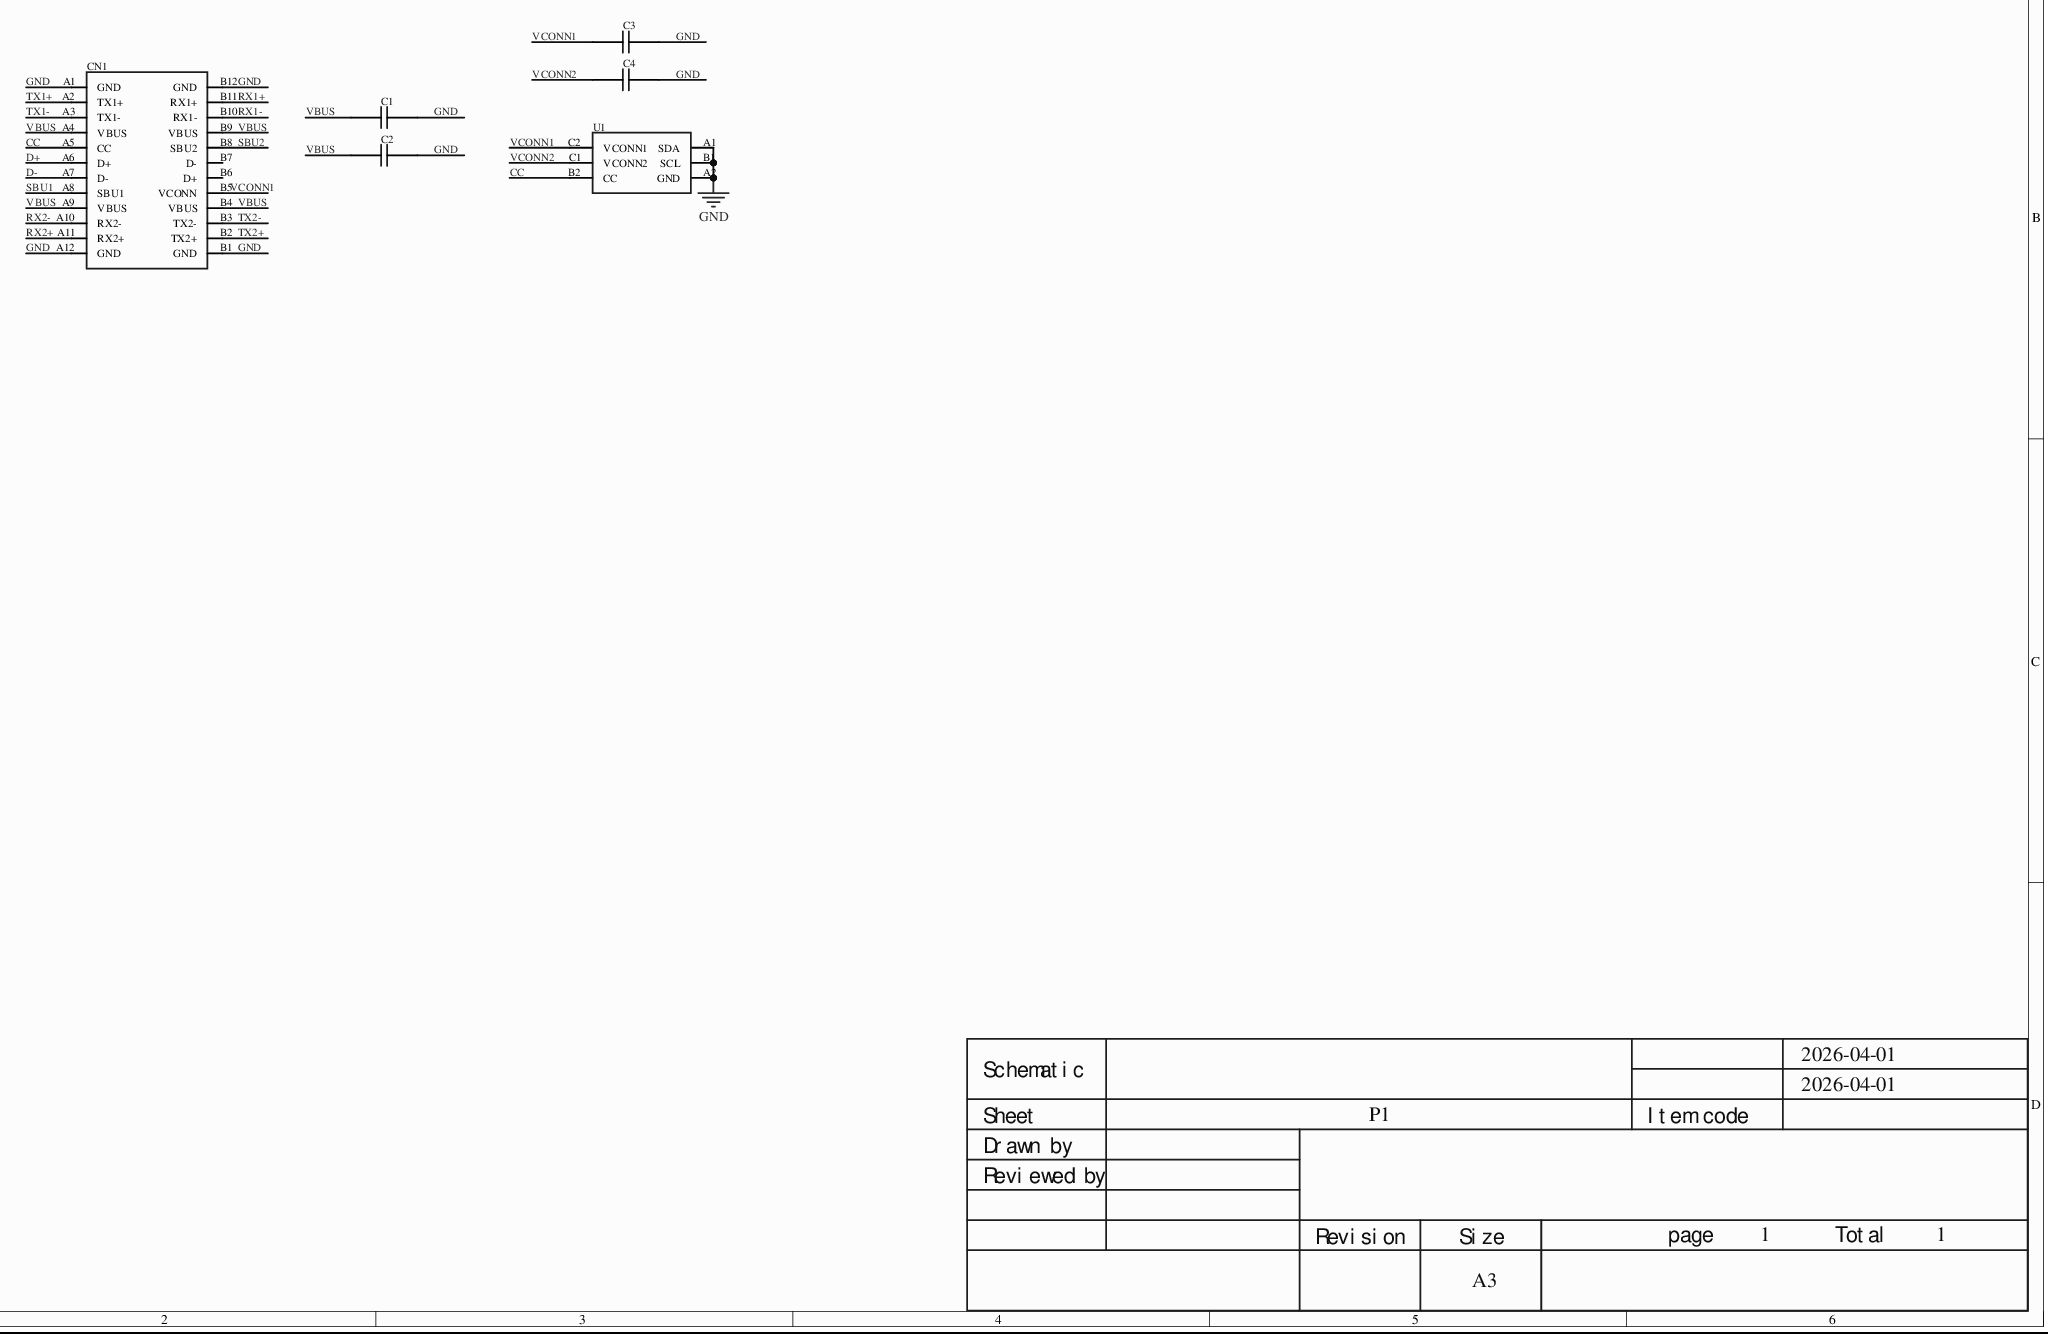
[diagram p0: MISC82881-3.schdoc]
# Altium project MISC82881-2.PrjPcb
1 sheet, 6 parts. Net scope: global (net labels, ports and power ports of the same name join across sheets).
Board file: MISC82881.pcbdoc

## Sheet MISC82881-3.schdoc
size 420 x 298 mm; Version: V1.0; @Project Name: MISC82881; @Page Count: 1; @Update Date: 2026-04-01; @Create Date: 2026-04-01; @Schematic Name: MISC82881; @Page No: 1

### Parts
C1  GRM022R61C104ME05  [c0201]  (value not drawn)
C2  GRM022R61C104ME05  [c0201]  (value not drawn)
C3  GRM022R61C104ME05  [c0201]  (value not drawn)
C4  GRM022R61C104ME05  [c0201]  (value not drawn)
CN1  (no value)  [简易版公头]
U1  (no value)  [wlcsp-6_l1.2-w0.8-r2-c3-p0.40-tl改]

### Nets
GND: C1.2 C2.2 C3.2 C4.2 CN1.A1(GND) CN1.A12(GND) CN1.B1(GND) CN1.B12(GND) U1.A1(SDA) U1.A2(GND) U1.B1(SCL)
CC: CN1.A5(CC) U1.B2(CC)
D+: CN1.A6(D+)
D-: CN1.A7(D-)
RX1+: CN1.B11(RX1+)
RX1-: CN1.B10(RX1-)
RX2+: CN1.A11(RX2+)
RX2-: CN1.A10(RX2-)
SBU1: CN1.A8(SBU1)
SBU2: CN1.B8(SBU2)
TX1+: CN1.A2(TX1+)
TX1-: CN1.A3(TX1-)
TX2+: CN1.B2(TX2+)
TX2-: CN1.B3(TX2-)
VBUS: C1.1 C2.1 CN1.A4(VBUS) CN1.A9(VBUS) CN1.B4(VBUS) CN1.B9(VBUS)
VCONN1: C3.1 CN1.B5(VCONN) U1.C2(VCONN1)
VCONN2: C4.1 U1.C1(VCONN2)

Not connected (* = marked no-connect by the designer): CN1 B6(D+)* B7(D-)*

### Notes on the sheet
- 2026-04-01
- Schematic
- Sheet
- P1
- Item code
- Reviewed by
- Drawn by
- Revision
- Size
- A3
- page
- 1
- Total

### Library data of the parts
C1-C4 = GRM022R61C104ME05: 3D Model: 1487c1e9cdde47f98c0de8937a3ba0c90819f05c4eef4c71ace90d822a990e87; AddInBom: yes; ModelName: C01005_L0.4-W0.2-H0.2; ModelTransform: 15.75,7.87,7.87,0,0,0,0,0,0; Device: GRM022R61C104ME05; ConvertToPcb: yes; SymbolName: GRM022R61C104ME05; FootprintName: c0201
CN1 = 简易版公头: Device: Simplified male header; SymbolName: Simplified male header; FootprintName: Simplified male header
U1 = 332B wlcsp-6: Device: 332B wlcsp-6; SymbolName: 332B wlcsp-6; FootprintName: wlcsp-6_l1.2-w0.8-r2-c3-p0.40-tl modified